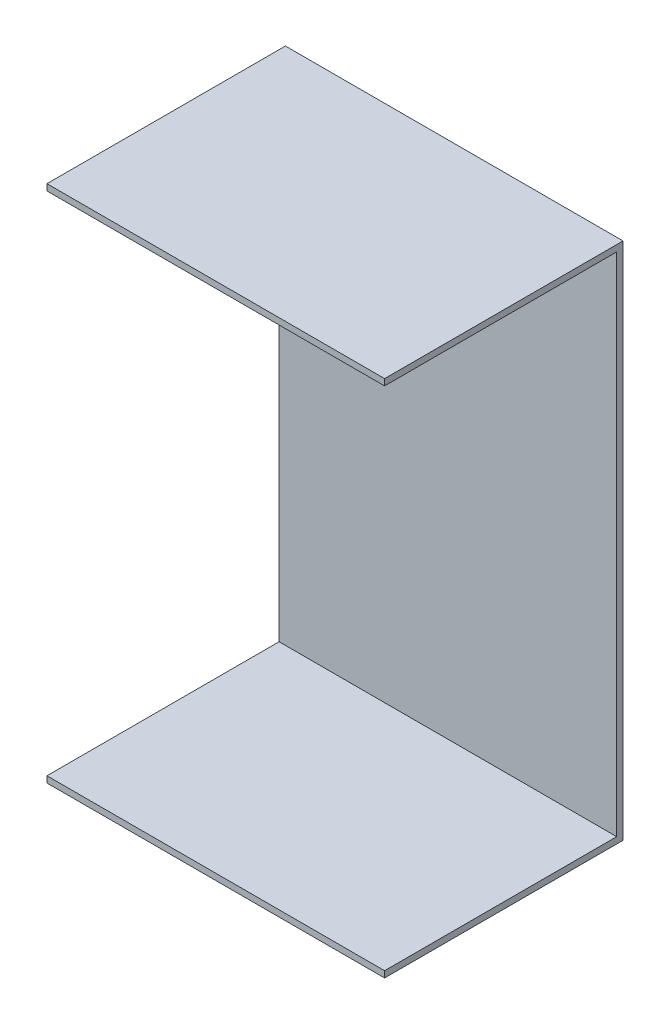
SolidWorks part; units mm, degrees
ref_plane "Front Plane" through (0, 0, 0) normal (0, 0, 1) x (1, 0, 0)
ref_plane "Top Plane" through (0, 0, 0) normal (0, 1, 0) x (1, 0, 0)
ref_plane "Right Plane" through (0, 0, 0) normal (1, 0, 0) x (0, 0, -1)
sketch "Sketch1" plane through (0, 0, 0) normal (0, 0, 1) x (1, 0, 0)
  line L1 (-80, 123) -> (80, 123)
  line L2 (-80, 123) -> (-80, -123)
  line L3 (-80, -123) -> (80, -123)
  line L4 (80, 123) -> (80, -123)
  line L5 (-80, 123) -> (80, -123) construction
  line L6 (-80, -123) -> (80, 123) construction
  point P0 (0, 0)
  dimension "D1" = 160
  dimension "D2" = 246
extrude "Boss-Extrude1" add sketch "Sketch1" along normal blind 3
sketch "Sketch2" plane through (0, 0, 3) normal (0, 0, 1) x (1, 0, 0)
  line L0 (80, -123) -> (80, 123) construction
  line L1 (-80, 123) -> (80, 123)
  line L2 (-80, 123) -> (-80, 120)
  line L3 (-80, 120) -> (80, 120)
  line L4 (80, 123) -> (80, 120)
  line L5 (-80, 123) -> (-80, -123) construction
  line L6 (80, -123) -> (-80, -123)
  line L7 (80, -123) -> (80, -120)
  line L8 (80, -120) -> (-80, -120)
  line L9 (-80, -123) -> (-80, -120)
  dimension "D1" = 3
  dimension "D2" = 3
extrude "Boss-Extrude2" add sketch "Sketch2" along normal blind 110
